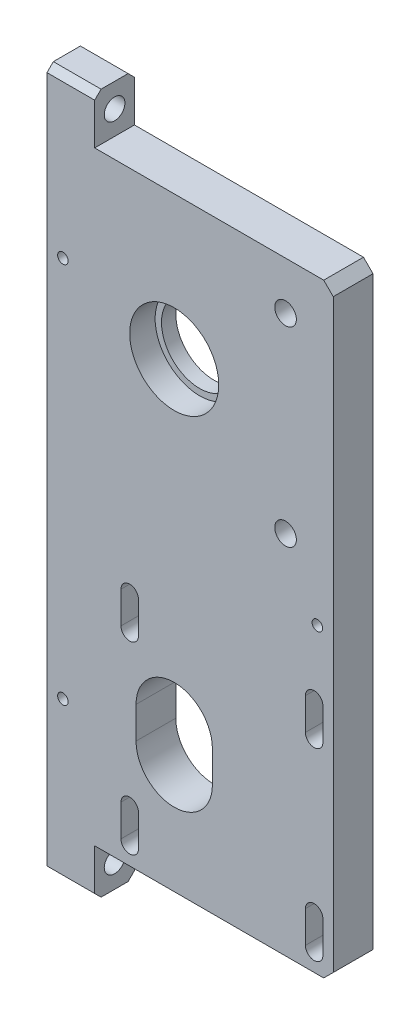
from build123d import *

# Parameters (mm, degrees)
SKETCH_1_W               = 90
SKETCH_1_H               = 220
EXTRUDE_1_DEPTH          = 12.5
SKETCH_2_R               = 12
CUT_EXTRUDE_1_DEPTH      = 239.025733903
HOLE_WIZARD_1_AT_2_COUNT = 2
HOLE_WIZARD_1_AT_2_PITCH = 57.982756057
HOLE_WIZARD_1_AT_3_COUNT = 2
HOLE_WIZARD_1_AT_3_PITCH = 82
HOLE_WIZARD_1_AT_4_COUNT = 2
HOLE_WIZARD_1_AT_4_PITCH = 57.982756057
HOLE_WIZARD_M4_1_D       = 3.3
CUT_EXTRUDE_5_DEPTH      = 239.025733903
CUT_EXTRUDE_6_DEPTH      = 6.5
SKETCH_14_R              = 12
CUT_EXTRUDE_7_DEPTH      = 239.025733903
SKETCH_15_R              = 14
CUT_EXTRUDE_8_DEPTH      = 8
HOLE_WIZARD_M8_1_D       = 6.8
SKETCH_19_W              = 12.5
SKETCH_19_H              = 15
CUT_EXTRUDE_10_DEPTH     = 75
CHAMFER_1_SIZE           = 2
CHAMFER_2_SIZE           = 3
SKETCH_20_R              = 3.25
CUT_EXTRUDE_11_DEPTH     = 233.76866198


with BuildPart() as part:
    # 草图1 → 凸台-拉伸1 (new body)
    with BuildSketch(Plane.XY):
        with Locations((-45, 110)):
            Rectangle(SKETCH_1_W, SKETCH_1_H)
    extrude(amount=EXTRUDE_1_DEPTH)

    # 草图2 → 切除-拉伸1 (cut, through all)
    with BuildSketch(Plane.XY.offset(12.5)):
        with Locations((-50, 55)):
            Circle(SKETCH_2_R)
    extrude(amount=-CUT_EXTRUDE_1_DEPTH, mode=Mode.SUBTRACT)

    # 草图3 → 打孔尺寸根据内六角圆柱头螺钉的类型1 (revolve, cut)
    with BuildSketch(Plane(origin=(-6.008621971, 83.991378029, 12.5), x_dir=(0, -1, 0), z_dir=(1, 0, 0))):
        Polygon((0, 0), (0, 12.5), (5, 12.5), (5, 6), (2.75, 6), (2.75, 0), align=None)
    hole_wizard_1 = revolve(axis=Axis((-6.008621971, 83.991378029, 18.85), (0, 0, -1)), mode=Mode.SUBTRACT)

    # 打孔尺寸根据内六角圆柱头螺钉的类型1 at 2: 打孔尺寸根据内六角圆柱头螺钉的类型1 ×2
    with Locations(*[(0, -i * HOLE_WIZARD_1_AT_2_PITCH, 0) for i in range(1, HOLE_WIZARD_1_AT_2_COUNT)]):
        add(hole_wizard_1, mode=Mode.SUBTRACT)

    # 打孔尺寸根据内六角圆柱头螺钉的类型1 at 3: 打孔尺寸根据内六角圆柱头螺钉的类型1 ×2
    with Locations(*[Vector(-0.7071067811865412, -0.7071067811865539, 0) * (i * HOLE_WIZARD_1_AT_3_PITCH) for i in range(1, HOLE_WIZARD_1_AT_3_COUNT)]):
        add(hole_wizard_1, mode=Mode.SUBTRACT)

    # 打孔尺寸根据内六角圆柱头螺钉的类型1 at 4: 打孔尺寸根据内六角圆柱头螺钉的类型1 ×2
    with Locations(*[(-i * HOLE_WIZARD_1_AT_4_PITCH, 0, 0) for i in range(1, HOLE_WIZARD_1_AT_4_COUNT)]):
        add(hole_wizard_1, mode=Mode.SUBTRACT)

    # M4 螺纹孔1 (through all)
    with Locations(Plane.XY.offset(12.5)):
        with Locations((-85, 170), (-85, 50), (-5, 110)):
            Hole(HOLE_WIZARD_M4_1_D / 2)

    # 草图12 → 切除-拉伸5 (cut, through all)
    with BuildSketch(Plane(origin=(0, 0, 0), x_dir=(-1, 0, 0), z_dir=(0, 0, -1))):
        with BuildLine():
            Line((38, 50), (38, 60))
            ThreePointArc((38, 60), (50, 72), (62, 60))
            Line((62, 60), (62, 50))
            ThreePointArc((62, 50), (50, 38), (38, 50))
        make_face()
        with BuildLine():
            Line((61.241378029, 78.991378029), (61.241378029, 88.991378029))
            ThreePointArc((61.241378029, 88.991378029), (63.991378029, 91.741378029), (66.741378029, 88.991378029))
            Line((66.741378029, 88.991378029), (66.741378029, 78.991378029))
            ThreePointArc((66.741378029, 78.991378029), (63.991378029, 76.241378029), (61.241378029, 78.991378029))
        make_face()
        with BuildLine():
            Line((66.741378029, 31.008621971), (66.741378029, 21.008621971))
            ThreePointArc((66.741378029, 21.008621971), (63.991378029, 18.258621971), (61.241378029, 21.008621971))
            Line((61.241378029, 21.008621971), (61.241378029, 31.008621971))
            ThreePointArc((61.241378029, 31.008621971), (63.991378029, 33.758621971), (66.741378029, 31.008621971))
        make_face()
        with BuildLine():
            Line((8.758621971, 31.008621971), (8.758621971, 21.008621971))
            ThreePointArc((8.758621971, 21.008621971), (6.008621971, 18.258621971), (3.258621971, 21.008621971))
            Line((3.258621971, 21.008621971), (3.258621971, 31.008621971))
            ThreePointArc((3.258621971, 31.008621971), (6.008621971, 33.758621971), (8.758621971, 31.008621971))
        make_face()
        with BuildLine():
            Line((8.758621971, 88.991378029), (8.758621971, 78.991378029))
            ThreePointArc((8.758621971, 78.991378029), (6.008621971, 76.241378029), (3.258621971, 78.991378029))
            Line((3.258621971, 78.991378029), (3.258621971, 88.991378029))
            ThreePointArc((3.258621971, 88.991378029), (6.008621971, 91.741378029), (8.758621971, 88.991378029))
        make_face()
    extrude(amount=-CUT_EXTRUDE_5_DEPTH, mode=Mode.SUBTRACT)

    # 草图13 → 切除-拉伸6 (cut)
    with BuildSketch(Plane(origin=(0, 0, 0), x_dir=(-1, 0, 0), z_dir=(0, 0, -1))):
        with BuildLine():
            Line((11.008621971, 88.991378029), (11.008621971, 78.991378029))
            ThreePointArc((11.008621971, 78.991378029), (6.008621971, 73.991378029), (1.008621971, 78.991378029))
            Line((1.008621971, 78.991378029), (1.008621971, 88.991378029))
            ThreePointArc((1.008621971, 88.991378029), (6.008621971, 93.991378029), (11.008621971, 88.991378029))
        make_face()
        with BuildLine():
            Line((68.991378029, 88.991378029), (68.991378029, 78.991378029))
            ThreePointArc((68.991378029, 78.991378029), (63.991378029, 73.991378029), (58.991378029, 78.991378029))
            Line((58.991378029, 78.991378029), (58.991378029, 88.991378029))
            ThreePointArc((58.991378029, 88.991378029), (63.991378029, 93.991378029), (68.991378029, 88.991378029))
        make_face()
        with BuildLine():
            Line((11.008621971, 31.008621971), (11.008621971, 21.008621971))
            ThreePointArc((11.008621971, 21.008621971), (6.008621971, 16.008621971), (1.008621971, 21.008621971))
            Line((1.008621971, 21.008621971), (1.008621971, 31.008621971))
            ThreePointArc((1.008621971, 31.008621971), (6.008621971, 36.008621971), (11.008621971, 31.008621971))
        make_face()
        with BuildLine():
            Line((68.991378029, 31.008621971), (68.991378029, 21.008621971))
            ThreePointArc((68.991378029, 21.008621971), (63.991378029, 16.008621971), (58.991378029, 21.008621971))
            Line((58.991378029, 21.008621971), (58.991378029, 31.008621971))
            ThreePointArc((58.991378029, 31.008621971), (63.991378029, 36.008621971), (68.991378029, 31.008621971))
        make_face()
    extrude(amount=-CUT_EXTRUDE_6_DEPTH, mode=Mode.SUBTRACT)

    # 草图14 → 切除-拉伸7 (cut, through all)
    with BuildSketch(Plane(origin=(0, 0, 0), x_dir=(-1, 0, 0), z_dir=(0, 0, -1))):
        with Locations((50, 160)):
            Circle(SKETCH_14_R)
    extrude(amount=-CUT_EXTRUDE_7_DEPTH, mode=Mode.SUBTRACT)

    # 草图15 → 切除-拉伸8 (cut)
    with BuildSketch(Plane.XY.offset(12.5)):
        with Locations((-50, 160)):
            Circle(SKETCH_15_R)
    extrude(amount=-CUT_EXTRUDE_8_DEPTH, mode=Mode.SUBTRACT)

    # M8 螺纹孔1 (through all)
    with Locations(Plane.XY.offset(12.5)):
        with Locations((-15, 130), (-15, 190)):
            Hole(HOLE_WIZARD_M8_1_D / 2)

    # 草图19 → 切除-拉伸10 (cut)
    with BuildSketch(Plane(origin=(0, 0, 0), x_dir=(0, 0, -1), z_dir=(1, 0, 0))):
        with Locations((-6.25, 212.5)):
            Rectangle(SKETCH_19_W, SKETCH_19_H)
        with Locations((-6.25, 7.5)):
            Rectangle(SKETCH_19_W, SKETCH_19_H)
    extrude(amount=-CUT_EXTRUDE_10_DEPTH, mode=Mode.SUBTRACT)

    # 倒角1
    chamfer_1_edges = [part.edges().sort_by_distance(p)[0] for p in [
        (-82.5, 220, 0),
        (-82.5, 220, 12.5),
        (-82.5, 0, 0),
        (-82.5, 0, 12.5),
    ]]
    chamfer(chamfer_1_edges, length=CHAMFER_1_SIZE)

    # 倒角2
    chamfer_2_edges = [part.edges().sort_by_distance(p)[0] for p in [
        (0, 205, 6.25),
        (0, 15, 6.25),
    ]]
    chamfer(chamfer_2_edges, length=CHAMFER_2_SIZE)

    # 草图20 → 切除-拉伸11 (cut, through all)
    with BuildSketch(Plane(origin=(-75, 0, 0), x_dir=(0, 0, -1), z_dir=(1, 0, 0))):
        with Locations((-6.25, 212.5)):
            Circle(SKETCH_20_R)
        with Locations(Location((-6.25, 7.5, 0), (0, 0, 180))):
            Circle(SKETCH_20_R)
    extrude(amount=-CUT_EXTRUDE_11_DEPTH, mode=Mode.SUBTRACT)


solid = part.part
